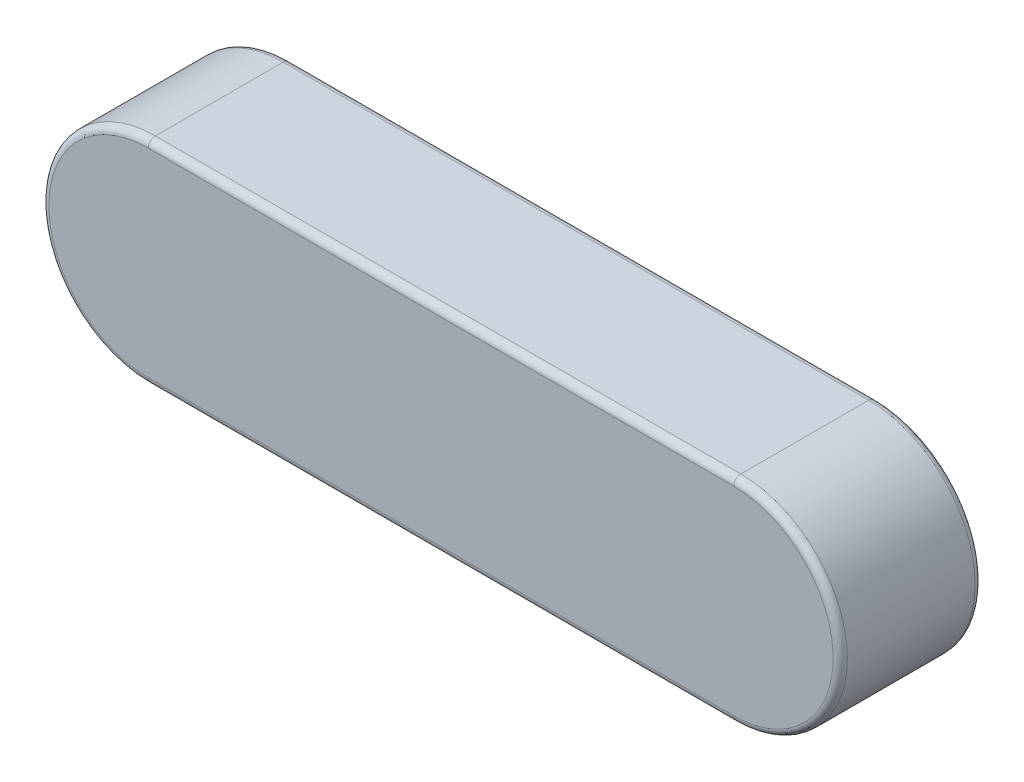
SolidWorks part; units mm, degrees
material "Steel"
ref_plane "Plane1" through (0, 0, 0) normal (0, 0, 1) x (1, 0, 0)
ref_plane "Plane2" through (0, 0, 0) normal (0, 1, 0) x (1, 0, 0)
ref_plane "Plane3" through (0, 0, 0) normal (1, 0, 0) x (0, 0, -1)
sketch "Dimension Sketch" plane through (0, 0, 0) normal (0, 0, 1) x (1, 0, 0)
  line L0 (-22.5, 0) -> (22.5, 0) construction
  point P3 (-8, 0)
  point P4 (0, 0)
  point P5 (0.4, 0)
  point P8 (-12, 0)
  point P11 (0, 0)
  dimension "L" = 45
  dimension "b" = 12
  dimension "h" = 8
  dimension "r" = 0.4
sketch "Sketch1" plane through (0, 0, 0) normal (0, 0, 1) x (1, 0, 0)
  line L0 (-22.5, 0) -> (22.5, 0) construction
  line L1 (-16.5, 6) -> (16.5, 6)
  line L2 (-16.5, -6) -> (16.5, -6)
  line L3 (0, 2.9108) -> (0, -6) construction
  arc A0 (-16.5, 6) -> (-16.5, -6) centre (-16.5, 0) ccw
  arc A1 (16.5, 6) -> (16.5, -6) centre (16.5, 0) cw
  dimension "D3" = 45
  dimension "D1" = 6
extrude "Boss-Extrude" add sketch "Sketch1" along normal blind 8
fillet "Fillet1" radius 0.4 8 edges at (22.5, 0, 8) (0, 6, 8) (-22.5, 0, 8) (0, 6, 0) (22.5, 0, 0) (0, -6, 0) (-22.5, 0, 0) (0, -6, 8)
